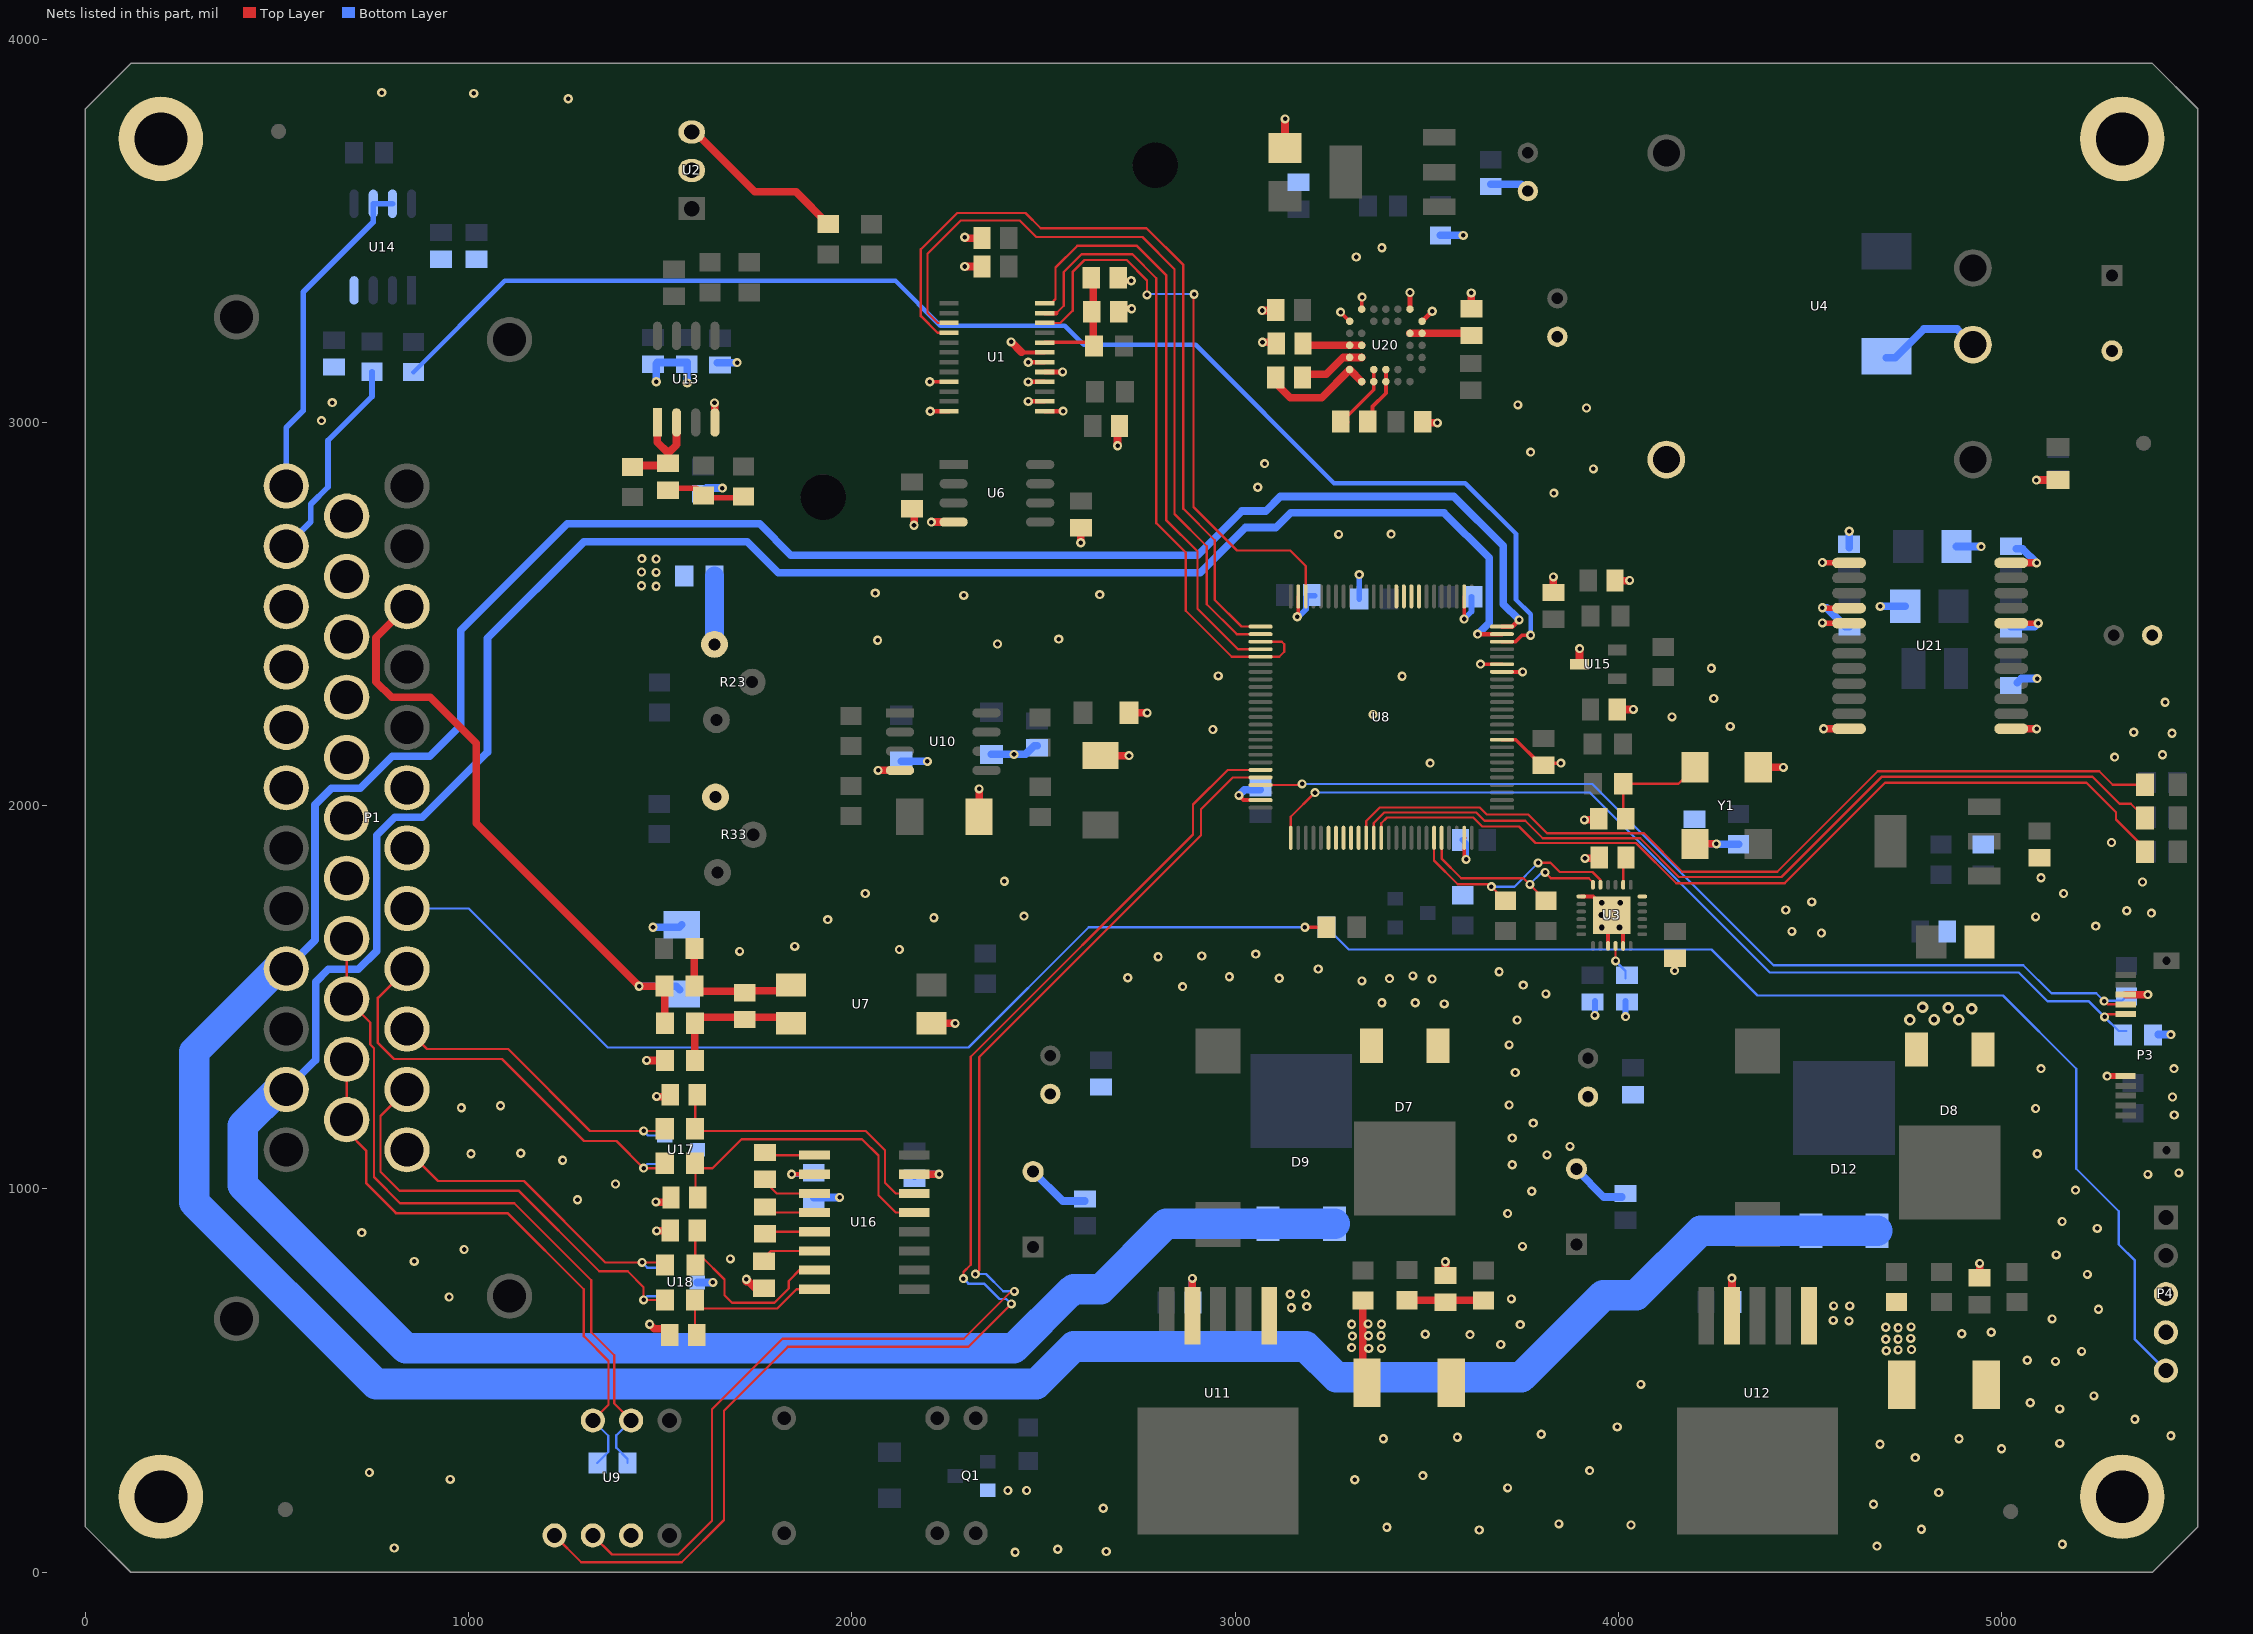
[diagram p0: the nets of this part, all layers, seen from the top]
# Altium PCB MISC82155.PcbDoc (part 3 of 5)
Units mil, origin at the board's own origin, x right, y up, seen from the top; angles counter-clockwise.
Board outline 5511.81 x 3937.01 mil, 4 copper layers (Top Layer, GND, POWER, Bottom Layer); 191 components, 134 nets, 709 pads, 440 vias.

## Via types
v1: diameter 24, hole 12, Top Layer to Bottom Layer, 278 vias
v2: diameter 23.62, hole 11.81, Top Layer to Bottom Layer, 144 vias
v3: diameter 30, hole 15, Top Layer to Bottom Layer, 17 vias
v4: diameter 20, hole 10, Top Layer to Bottom Layer, 1 vias

## Nets (pads, with @x,y where several pads share a name; then routed paths per layer and width w, separated by ;. In a path a pad name is that pad's centre, name@x,y a point inside that pad or via, vN(x,y) a via of type N, cw(c..) or ccw(c..) an arc to the next point about the centre after c; other vN are vias at no path point) (continued)
6050_SCL: R42.1 U3.23 U8.95 | length 630.8
  Top Layer w6: U8.95@3519.2,1916.38 3519.2,1856.8 3581,1795 3662.5,1795 v2(3668.75,1788.75) R42.1@3705.32,1752.18 ; v2(3791,1851) 3823,1851 3847,1827 3933,1827 3953.47,1806.53 U3.23@3953.47,1793.72
  Bottom Layer w6: v2(3668.75,1788.75) 3728.75,1788.75 v2(3791,1851)
6050_SDA: R41.1 U3.24 U8.96 | length 567.4
  Top Layer w6: U8.96@3538.89,1916.38 3538.89,1862.11 3590,1811 3752.5,1811 v2@3768.75,1794.75 ; v2(3769,1795) v2@3768.75,1794.75 ; v2(3809,1826) 3824,1811 3923,1811 3933.79,1800.21 U3.24@3933.79,1793.72 ; R41.1@3811.32,1752.18 v2@3768.75,1794.75
  Bottom Layer w6: v2(3769,1795) 3800,1826 v2(3809,1826)
ACC_INT1: U8.35
ACC_INT2: U8.36
AD_INA: R2.2 U2.3 | length 455.9
  Top Layer w20: U2.3@1582,3758 1591,3758 1747,3602 1854.12,3602 R2.2@1938.41,3517.71
AD_MISO: U1.23 U8.53 U8.55 | length 1728.2
  Top Layer w6: 2533.56,3285.5 2553,3304.93 2553,3393 2599,3439 2732,3439 2794.41,3376.59 2794.41,2737.59 2871,2661 2871,2509 2991.18,2388.82 U8.55@3066.45,2388.82 3115.41,2388.82 3128.41,2401.82 3128.41,2421.34 3121.56,2428.19 U8.53@3066.45,2428.19
  Top Layer w11.81: U1.23@2503.41,3285.5 2533.56,3285.5
AD_MOSI: U1.24 U8.54 | length 1571.4
  Top Layer w6: U1.24@2503.41,3311.09 2520.15,3311.09 2531.41,3322.34 2531.41,3404.41 2588,3461 2744,3461 2820,3385 2820,2746 2902,2664 2902,2514 3007.49,2408.51 U8.54@3066.45,2408.51
AD_NSS: U1.4 U8.51 | length 2102.5
  Top Layer w6: U1.4@2253.41,3234.32 2223.43,3234.32 2180,3277.75 2180,3452 2275,3547 2453,3547 2493,3507 2769,3507 2865,3411 2865,2775 2947,2693 2947,2537 3016.44,2467.56 U8.51@3066.45,2467.56
AD_SCK: U1.3 U8.52 | length 2035.6
  Top Layer w6: U1.3@2253.41,3259.91 2223.84,3259.91 2197.41,3286.34 2197.41,3440.34 2284.07,3527 2438,3527 2481,3484 2758,3484 2842,3400 2842,2761 2926,2677 2926,2526 3004.12,2447.88 U8.52@3066.45,2447.88
AD_SYNC: U1.22 U8.48 | length 1567.8
  Top Layer w6: U1.22@2503.41,3259.91 2543.97,3259.91 2576,3291.93 2576,3393 2607,3424 2717,3424 2770,3371 v1(2770,3333) ; v1@2891.41,3333.41 2891.41,2779.59 3005,2666 3144,2666 3184.56,2625.44 U8.48@3184.56,2546.3
  Bottom Layer w6: v1(2770,3333) 2772.34,3335.34 2892.66,3335.34 v1(2893,3335)
AGND: C3.2 C4.2 C5.2 C11.1 C13.2 C29.2 C30.2 C39.1 C72.2 C73.2 C74.2 C75.2 D4.1 D10.1 D11.1 DW3.1 DW4.1 R4.1 R12.2 R23.1 R33.1 U1.9 U1.12 U1.13 U1.14 U1.16 U1.17 U1.18 U2.2 U6.4 U13.4 U20.F1 U20.G2 | length 1766.4
  Top Layer w10: v1@2204.43,3106.36 U1.9@2253.41,3106.36 ; v1@2460.15,3157.55 v1@2460.41,3157.55
  Top Layer w12: v1(2204.66,3029.59) U1.12@2253.41,3029.59 ; v2(2460.18,3055.18) U1.14@2503.41,3055.18 ; v1@2460.15,3106.36 U1.16@2503.41,3106.36 ; v1@2460.41,3157.55 U1.18@2503.41,3157.55 ; U1.13@2503.41,3029.59 v2(2551.41,3029.59) ; U1.17@2503.41,3131.96 v2(2549.96,3131.96) ; U20.G2@3456.4,3295.83 v1@3456.4,3337.34 ; U20.F1@3487.89,3264.33 v1@3514.15,3290.59
  Top Layer w15: v1@2206,2739 v1(2207.34,2740.34) ; C4.2@2688.93,3297.34 2729.66,3297.34 v1(2730,3297) ; C5.2@2688.93,3370.34 2728.66,3370.34 v1(2729,3370)
  Top Layer w20: v2(1464.34,1335.34) R12.2@1512.04,1335.34 ; v1(1641.41,3051.34) 1642.41,3050.34 U13.4@1642.41,3000.34 ; v1(2162,2732) 2162.41,2732.41 C11.1@2162.41,2780.81 ; v1@2204.41,3029.34 v1(2204.66,3029.59) ; v1(2207.34,2740.34) U6.4@2265.41,2740.34 ; D10.1@2331.96,1971.34 v2(2331.96,2043.96) ; v1(2597.41,2686.34) C13.2@2597.41,2730.81 ; D11.1@2648.41,2130.89 v2(2723.11,2130.89) ; v1@2692.93,2939.81 C3.2@2692.93,2991.34 ; DW4.1@2723.41,2242.34 v2(2770.34,2242.34) ; v1(3070.41,3292.34) C39.1@3113.88,3292.34
  Bottom Layer w20: v2(1481,1683) 1549.45,1683 D4.1@1556,1689.55 ; v1(1489.41,3106.34) 1489.41,3153.81 1492.41,3156.81 1570.41,3156.81 1570.41,3110.34 v2(1570.41,3103.59) ; C72.2@1611,2819.47 1620.53,2829 v2(1662,2829) ; C73.2@1649,3156.47 v2(1700.53,3156.47) ; DW3.1@2129,2116 v2(2197,2116) ; C30.2@2364,2134 v2(2423,2134) 2453,2134 2475.47,2156.47 C29.2@2483,2156.47
  Bottom Layer w50: R23.1@1641.37,2421.23 R4.1@1641.37,2600
  other v1: 2693.41,2939.34 2203.41,3106.34 2460.41,3106.11 2460.41,3157.29 3514.41,3290.34 3456.4,3339.34
ANG_INA: R54.2 U8.23 | length 3611.6
  Top Layer w10: U8.23@3696.37,2428.19 3732.19,2428.19 3749,2445 v2(3771,2445)
  Bottom Layer w12: R54.2@856,3131.63 1094.54,3370.17 2113.83,3370.17 2231,3253 2555,3253 2605,3203 2897,3203 3258,2842 3601,2842 3733,2710 3733,2538 3771,2500 v2(3771,2445)
ANG_R+: P1.24 U14.6 U14.7 | length 880.5
  Bottom Layer w15: P1.24@524.03,2834.48 524.03,2987.03 568,3031 568,3340 751,3523 U14.6@751,3571 U14.7@801,3571
ANG_R-: P1.25 R61.2 | length 548.4
  Bottom Layer w15: P1.25@524.03,2677 588,2740.97 588,2787 633,2832 633,2953 748,3068 R61.2@748,3132.63
AVDD1: C4.1 C5.1 L1.2 U1.20 | length 286.9
  Top Layer w10: U1.20@2504.02,3209.34 L1.2@2630.04,3209.34
  Top Layer w20: L1.2@2629.88,3209.5 2629.88,3297.34 C5.1@2629.88,3370.34
BOOT0: P1.8 P4.5 R34.2 R55.1 | length 5730.9
  Top Layer w10: v2(3182,1683) R55.1@3238.63,1683
  Bottom Layer w6: P1.8@838.99,1732.12 999.88,1732.12 1363,1369 2304,1369 2618,1683 v2(3182,1683) R34.2@3238.63,1683 3296.63,1625 4243,1625 4363,1505 5004,1505 5195,1314 5195,1111 5195,1053 5306,942 5306,855 5348,813 5348,607 P4.5@5429,526
CAN0_RXD: U8.70 U9.1 | length 3518.5
  Top Layer w6: U9.1@1224,96 1294,26 1556,26 1666,136 1666,421 1833,588 2304,588 v2(2416,700) ; v2(2291,766) 2291,783 2310,802 2310,1345 2890,1925 2890,2003 2980.55,2093.55 U8.70@3066.45,2093.55
  Bottom Layer w6: v2(2291,766) 2304,753 2345,753 2385,713 2403,713 v2(2416,700)
CAN0_TXD: U8.71 U9.2 | length 3345.1
  Top Layer w6: U9.2@1324,96 1374,46 1547,46 1635,134 1635,425 1819,609 2292,609 2416,733 v2(2424,733) ; v2(2322,778) 2322,777 2332,787 2332,1344 2911,1923 2911,1991 2993.86,2073.86 U8.71@3066.45,2073.86
  Bottom Layer w6: v2(2322,778) 2350,778 2395,733 v2(2424,733)
CANH: P1.22 P1.23 R40.1 U9.7 | length 1566.3
  Top Layer w6: P1.22@681.51,1338.42 P1.23@681.51,1180.94 681.51,1150.49 733,1099 733,1014 810,937 1101,937 1300,738 1300,665 ; 1300,651 1300,665 ; U9.7@1324,396 1365,437 1365,551 1300,616 1300,665
  Bottom Layer w6: U9.7@1324,396 1364,356 1364,313.37 R40.1@1335.63,285
CANL: P1.20 P1.21 R40.2 U9.6 | length 1878.8
  Top Layer w6: P1.20@681.51,1653.38 P1.21@681.51,1495.9 743,1434.41 743,1377 753,1367 753,1031 821,963 1119,963 1320,762 1320,626 1380,566 1380,440 U9.6@1424,396
  Bottom Layer w6: R40.2@1414.37,285 1414.37,295.63 1385,325 1385,357 U9.6@1424,396
COM1_RXD: P1.11 R59.2 U18.1 | length 1203
  Top Layer w6: P1.11@838.99,1259.68 770,1190.69 770,1045 820,995 1131,995 1341,785 1415,785 1456.34,743.66 v2(1456.34,710.34) R59.2@1512.04,710.34
  Bottom Layer w6: v2(1456.34,710.34) 1465.94,719.94 U18.1@1511.91,719.94
COM1_TXD: P1.12 R58.2 U18.2 | length 860
  Top Layer w6: P1.12@838.99,1102.2 920.19,1021 1144,1021 1356.66,808.34 v2(1452.34,808.34) R58.2@1512.04,808.34
  Bottom Layer w6: v2(1452.34,808.34) 1465.94,794.74 U18.2@1511.91,794.74
COM2_RXD: P1.9 R57.2 U17.1 | length 1169.4
  Top Layer w6: P1.9@838.99,1574.64 763,1498.65 763,1381 805,1339 1087,1339 1301,1125 1385.68,1125 v2(1456.34,1054.34) R57.2@1512.04,1054.34
  Bottom Layer w6: v2(1456.34,1054.34) 1466.94,1064.94 U17.1@1511.91,1064.94
COM2_TXD: P1.10 R56.2 U17.2 | length 843.5
  Top Layer w6: P1.10@838.99,1417.16 891.15,1365 1103,1365 1316.66,1151.34 v2(1456.34,1151.34) R56.2@1512.04,1151.34
  Bottom Layer w6: v2(1456.34,1151.34) 1467.94,1139.74 U17.2@1511.91,1139.74
FOOT_SW: D4.2 P1.3 R6.1 R8.1 | length 1653.8
  Top Layer w20: P1.3@853.48,2519.52 P1.3@838.99,2519.52 758,2438.53 758,2324 799,2283 900,2283 1020,2163 1020,1954 v2@1444.66,1529.34 ; v2(1445,1529) v2@1444.66,1529.34 ; R8.1@1511.04,1529.34 v2@1444.66,1529.34 ; R6.1@1512.04,1432.34 R8.1@1512.04,1528.34
  Bottom Layer w20: v2(1445,1529) 1541.3,1529 D4.2@1550.41,1519.89
GND: C1.2 C6.2 C7.1 C8.2 C9.1 C10.2 C12.1 C14.2 C15.2 C17.1 C18.2 C19.2 C21.2 C22.2 C23.2 C24.2 C25.2 C26.2 C27.2 C28.1 C31.2 C32.2 C33.2 C34.2 C35.2 C36.1 C37.1 C40.2 C41.1 C42.1 C43.2 C44.1 C46.2 C47.2 C48.2 C50.2 C51.2 C52.2 C53.2 C54.1 C55.1 C56.1 C57.2 C61.2 C62.2 C63.2 C64.2 C65.2 C66.2 C67.2 C68.2 C69.2 C70.1 C76.2 C77.2 C78.2 D5.2 D6.1 D7.1 D8.1 H1.8 H2.8 H3.8 H4.8 P1.6 P1.7 P1.13 P1.14 P1.15 P1.16 P1.17 P1.18 P1.19 P1.26 P1.27 P1.28 P1.29 P3.5 P3.8 P4.3 P4.4 Q1.2 R4.2 R13.1 R20.1 R21.1 R27.1 R28.1 R38.1 R44.1 U1.19 U3.1 U3.9 U3.11 U3.18 U4.2 U4.5 U7.3 U8.10 U8.19 U8.20 U8.27 U8.49 U8.74 U8.99 U9.3 U10.4 U11.1 U12.1 U14.4 U15.3 U16.15 U17.3 U18.3 U20.F7 U20.G6 U21.1 U21.8 U21.12 U21.13 U21.16 U21.17 U21.24 Y1.2 | length 4636.4
  Top Layer w6: v2(3597.41,2487.34) v2@3597.94,2487.88
  Top Layer w9: v2@3597.94,2487.88 U8.27@3597.94,2546.3
  Top Layer w10: 2442.61,3183.14 U1.19@2503.41,3183.14 ; v2(3010,2027) 3022.19,2014.81 U8.74@3066.45,2014.81 ; v1(3162.41,2493.34) 3162.41,2496.34 3164.87,2498.81 U8.49@3164.87,2546.3 ; v1@3275.41,3287.85 U20.F7@3298.92,3264.33 ; U20.G6@3330.41,3295.83 v1@3330.41,3326.35 ; U8.99@3598.41,1915.92 U8.99@3597.94,1916.38 3597.94,1865.06 v2(3603,1860) ; v2(3640.41,2369.34) 3640.61,2369.14 U8.20@3696.37,2369.14 ; U8.10@3696.37,2172.29 3732.46,2172.29 3793.93,2110.81 3849.88,2110.81 v2(3850.41,2111.34) ; U8.19@3696.37,2349.45 3750.3,2349.45 v2(3750.41,2349.34) ; U3.1@3903.28,1763.21 3933.79,1763.21 U3.1@3983,1714 3973.16,1704.16 U3.9@3973.16,1634.28 ; U3.11@4012.53,1634.28 U3.1@4012.53,1684.47
  Top Layer w15: U3.1@3983,1714 U3.1@4012.53,1684.47 ; v2(4147,1570) 4147,1606.47 C41.1@4148,1607.47 ; v1@4533.61,2476.35 U21.17@4602.17,2476.35 ; v1@4533.61,2515.72 U21.16@4602.17,2515.72 ; v1@4533.61,2633.83 U21.13@4602.17,2633.83 ; U21.8@5025.4,2476.35 v1(5095.66,2476.41) ; v2(5275.35,1294.65) P3.5@5323.46,1294.65
  Top Layer w20: v2(1472,647) 1484,635 C50.2@1535,635 ; v2(1488.41,966.34) 1489.41,965.34 C52.2@1532.88,965.34 ; v2(1490.41,890.34) 1491.41,891.34 C51.2@1531.88,891.34 ; v2(1490.41,1241.34) 1491.41,1240.34 C53.2@1531.88,1240.34 ; v2@1724.93,758.34 v2@1730.41,758.34 ; v2@1724.93,763.81 v2(1724.41,764.34) v2@1730.41,758.34 ; C48.2@1771,741 1747.75,741 v2@1730.41,758.34 ; v2(2068.34,2092.34) U10.4@2125.41,2092.34 ; U16.15@2162.41,1038.34 v2(2227.41,1038.34) ; U7.3@2207.48,1432.34 v2(2269.41,1432.34) ; v1@2295.41,3481.34 C14.2@2344.88,3481.34 ; v1@2296.41,3407.34 C15.2@2344.88,3407.34 ; v1(2415.41,3210.34) 2442.61,3183.14 ; v1@3072.41,3209.34 C56.1@3114.88,3209.34 ; C6.2@3130.41,3716.33 v1@3130.41,3791.34 ; C44.1@3483.93,2999.34 v2(3527.66,2999.34) ; C32.2@3549,768.53 v2(3549,810) ; C57.2@3616.41,3291.87 v1(3616.41,3338.34) ; C37.1@3830.41,2550.87 v2(3830.41,2597.34) ; U15.3@3898.79,2369 v2(3898.79,2409.79) ; v2(3911.41,1963.34) C28.1@3954.88,1963.34 ; v2(3913.07,1862.75) C55.1@3955.54,1862.75 ; C36.1@3985.93,2587.34 4028.41,2587.34 v2(4029.41,2588.34) ; C17.1@3991.93,2251.34 v2(4039.41,2251.34) ; Y1.2@4365.08,2100.34 v2(4430.66,2100.34) ; v2(4536,2201) 4536.24,2200.76 U21.24@4602.17,2200.76 ; C69.2@4943,762.53 v2(4943,806) ; U21.1@5025.4,2200.76 v2(5091.76,2200.76) ; U21.12@5025.4,2633.83 v2(5091.83,2633.83) ; v2(5091.03,2850.03) D5.2@5147.41,2850.03 ; P3.8@5324.16,1507.25 v2(5381.75,1507.25)
  Bottom Layer w15: v1(3162.41,2493.34) 3165.34,2493.34 3185,2513 3185,2544 3189.34,2548.34 C27.2@3207.93,2548.34 ; R20.1@3324.04,2539.34 v2(3324.04,2602.96) ; C26.2@3593.47,1911 3603,1901.47 v2(3603,1860) ; v2(3597.41,2487.34) 3616.93,2506.87 C24.2@3616.93,2545.34 ; v2(3939,1453) C42.1@3939,1490.47 ; v2(4019,1450) C54.1@4019,1490.47
  Bottom Layer w20: U18.3@1596.5,756 v2(1637,756) ; C47.2@1900.41,977.81 v2(1968.19,977.81) ; C46.2@2163.41,1033.81 2167.93,1038.34 v2(2227.41,1038.34) ; C18.2@2473,1045.43 2549.9,968.53 C19.2@2608,968.53 ; v2(3010,2027) 3024.53,2041.53 C25.2@3066,2041.53 ; R21.1@3536,3488.63 v2(3595.37,3488.63) ; C7.1@3667,3621.47 3746.53,3621.47 C1.2@3764,3604 ; C33.2@3891,1052.43 3891,1049.87 3962,978.87 C34.2@4009.41,978.87 ; v1(4532.66,2516.67) 4543.33,2516.67 4593,2467 C65.2@4603,2467 ; C63.2@4602.66,2672.93 v2(4602.66,2716.34) ; v2(4683.59,2520.41) C62.2@4748.67,2520.41 ; D6.1@4700,3169.19 4722.19,3169.19 4797,3244 4884.75,3244 U4.2@4925.41,3203.34 ; C61.2@4882.65,2676.41 v2(4946.59,2676.41) ; C64.2@5024.66,2466.88 5086.13,2466.88 v1(5095.66,2476.41) ; C66.2@5038.73,2671 5054.66,2671 v2(5091.83,2633.83) ; C67.2@5041,2321 5051.88,2331.88 v2(5092.88,2331.88) ; R44.1@5409.37,1403 v2(5442,1403)
  other v1: 2426,52 2664,54 2537,60 806,63 4675,68 5159,73 3637,110 4791,112 3396,117 4033,123 3845,126 2656,167 4666,177 4836,208 2407,213 2456,213 3711,220 3312,241 952,242 3490,252 741,260 3925,265 4775,299 5000,322 4683,334 5152,336 3387,348 4889,348 3580,352 5442,356 3799,360 3997,379 5348,399 5152,426 5075,442 5241,460 4059,490 5141,550 5067,553 5209,576 3693,594 3613,620 3496,621 4896,622 4973,626 3744,646 4561,657 5132,661 5253,686 3147,690 3187,693 3721,713 949,718 3144,725 3184,726 5224,777 858,811 5143,828 988,842 3750,850 721,886 5250,897 5158,915 3711,936 1284,972 3774,994 5193,997 1383,1013 5382,1038 5463,1042 3723,1063 1245,1075 3814,1089 1006,1092 5093,1092 1136,1093 3874,1111 3723,1133 3778,1172 5451,1193 5089,1210 981,1212 1083,1217 3715,1219 5446.19,1240 3731,1304 5103,1314 5450.19,1314 3715,1376 3736,1441 3546,1483 3383,1486 3470,1486 3811,1509 2863,1528 3752,1532 3331,1543 3514,1548 3403,1549 3115,1550 2720,1551 2985,1554 3464,1556 3689,1567 3217,1574 2799,1606 2913,1608 3054,1613 1707,1620 2124,1625 1851,1633 4530,1668 4453,1672 5246,1686 1937,1703 2214,1708 5089,1710 2449,1712 5391,1720 5327,1726 4437,1728 4505,1749 2035,1771 5162,1771 5368,1801 2398,1803 5103,1812 5287,1904 5295,2127 5420,2133 5445,2189 5345,2192 2942,2199 4292,2207 4140,2232 5427,2270 4249,2280 2956,2339 4243,2359 2380,2422 2067,2432 2540,2435 4532.66,2477.3 2292,2549 2647,2551 2061,2555 1489,2573 1451,2574 1489,2609 1451,2610 4532.66,2634.78 1489,2644 1452,2645 3270,2708 3407,2709 3832,2816 3059,2831 3935,2879 3077,2893 3771,2923 616,3005 3917,3038 3738,3046 644,3052 3071.41,3209.34 3275.41,3288.34 3331.41,3327.34 2294.41,3407.34 3316,3432 3383,3456 2294.41,3483.34 3130.41,3792.34 1260,3845 1013,3859 773,3861
  other v2: 4602,656 4562,695 4604,695 1682.93,817.81 3509,2111 3360,2238 3436,2338
  other v3: 4761,1441 4889,1441 4824,1442 4922,1470 4861,1473 4794,1474 3957,1682 4003,1682 3956,1715 3957,1747 4005,1747
GND_SA: D9.1 P1.34 R13.2 R16.1 U8.24 | length 8267.6
  Top Layer w12: v2(3633.12,2447.88) U8.24@3696.37,2447.88
  Top Layer w20: R13.2@3333.17,532.34 R16.1@3333.17,707.8
  Bottom Layer w20: P1.34@524.03,1259.68 601,1336.65 601,1540 634,1573 712,1573 760,1621 760,1923 807,1970 879,1970 1049,2140 1049,2437 1301,2689 1727,2689 1808,2608 2909,2608 3027,2726 3106,2726 3145,2765 3545,2765 3663,2647 3663,2477.75 v2(3633.12,2447.88)
  Bottom Layer w80: P1.34@524.03,1259.68 504.68,1259.68 410,1165 410,1010 836,584 2422,584 2570,732 2572.02,732 2578.52,738.5 2649.5,738.5 2820,909 D9.1@3086.39,909 D9.1@3259.61,909
  other v1: 3349,584 3382,584 3304,586 3306,616 3348,617 3381,617 3304,647 3382,647 3347,648
GND_SB: D12.1 P1.32 R26.1 R27.2 U8.25 | length 10109
  Top Layer w12: U8.25@3696.37,2467.56 3723.56,2467.56 v2(3741,2485)
  Bottom Layer w20: P1.32@524.03,1574.64 599.08,1649.7 599.08,1920.69 599,1920.77 599,2003 642,2046 717,2046 800.51,2129.51 898.51,2129.51 979,2210 979,2458 1257,2736 1759,2736 1841,2654 2902,2654 3017,2769 3080,2769 3118,2807 3571,2807 3700,2678 3700,2526 v2(3741,2485)
  Bottom Layer w80: P1.32@524.03,1574.64 500.64,1574.64 284,1358 284,965 758,491 2481,491 2579,589 3184,589 3264,509 3531,509 ; 3675.34,509 3531,509 ; D12.1@4675.61,891 D12.1@4502.39,891 4215,891 4047,723 3961,723 3747,509 3531,509
  other v1: 4699,578 4730,580 4765,581 4698,608 4730,608 4763,610 4730,638 4698,639 4764,640
GYRO_INT1: U8.34
GYRO_INT2: U8.33
JTCK: P3.6 R44.2 U8.76 | length 2577.8
  Top Layer w6: U8.76@3145.19,1916.38 3145.19,1971.19 v2(3208.5,2034.5) ; v2(5269,1449) 5276.07,1456.07 P3.6@5324.16,1456.07
  Bottom Layer w6: v2(3208.5,2034.5) 3925.5,2034.5 4395,1565 5045,1565 5120.5,1489.5 5228.5,1489.5 v2(5269,1449) 5306,1412 R44.2@5326,1412
JTMS: P3.7 R45.2 U8.72 | length 2549.2
  Top Layer w6: U8.72@3066.45,2054.18 3164.18,2054.18 3167,2057 v2(3175,2057) ; v2@5276.34,1481.66 P3.7@5324.16,1481.66
  Bottom Layer w6: v2(3175,2057) 3932,2057 4405,1584 5057,1584 5130.5,1510.5 5247.5,1510.5 v2@5267,1491 ; v2(5268,1490) v2@5267,1491 ; R45.2@5326,1502.63 5314.37,1491 v2@5267,1491
LED_O1: D1.2 U8.88 | length 2307.4
  Top Layer w6: U8.88@3381.41,1916.38 3381.41,1954.34 3396.41,1969.34 3621.41,1969.34 3644.75,1946 3741,1946 3784,1903 4046,1903 4151,1798 4434,1798 4696,2060 5222,2060 5299,1983 5299,1964 5374.39,1888.61 D1.2@5374.39,1880
LED_O2: D2.2 U8.87 | length 2285.4
  Top Layer w6: U8.87@3361.72,1916.38 3361.72,1954.66 3389.41,1982.34 3629.41,1982.34 3650.75,1961 3757,1961 3803,1915 4057,1915 4158,1814 4426,1814 4688,2076 5237,2076 5308,2005 5337.39,2005 D2.2@5374.39,1968
LED_O3: D3.2 U8.86 | length 2282.9
  Top Layer w6: U8.86@3342.04,1916.38 3342.04,1959.97 3377.41,1995.34 3638.41,1995.34 3656.75,1977 3765,1977 3814,1928 4067,1928 4167,1828 4415,1828 4677,2090 5255,2090 5290,2055 D3.2@5374.39,2055
LED_O4: U8.85
LED_O5: U8.84
LED_O6: U8.83
LED_O7: U8.82
LED_O8: U8.81
NetC2_1: C2.1 R39.1 U13.1 U13.2 | length 319
  Top Layer w20: R39.1@1416,2884.37 1419.5,2887.87 C2.1@1520.41,2887.87 ; U13.1@1492.41,3000.34 1492.41,2948.59 1520.41,2920.59 ; C2.1@1520.25,2887.71 C2.1@1520.41,2887.87 ; U13.2@1542.41,3000.34 1542.41,2942.59 1520.41,2920.59 ; C2.1@1520.41,2887.87 1520.41,2920.59
NetC2_2: C2.2 R43.2 R46.1 | length 239.1
  Top Layer w11.81: R46.1@1588.56,2828.81 R46.1@1609.41,2807.97 ; R43.2@1708.41,2807.97 R43.2@1709.41,2806.97
  Top Layer w15: C2.2@1520.41,2828.81 1593.82,2828.81 1618.94,2803.69 1714.06,2803.69 R43.2@1717,2806.63
NetC16_1: C16.1 R8.2 R11.1 U7.1 | length 369.8
  Top Layer w19.68: R11.1@1588.78,1627.34 1588.78,1530.34 1602.78,1516.34 1710.93,1516.34 1720.41,1506.87 1730.88,1517.34 1826.34,1517.34 U7.1@1841.34,1532.34
NetC16_2: C16.2 R6.2 R12.1 U7.2 | length 364
  Top Layer w19.68: R12.1@1590.78,1331.34 1589.78,1332.34 1589.78,1429.34 1608.25,1447.81 1825.86,1447.81 U7.2@1841.34,1432.34
NetC20_2: C20.2 U11.4 | length 178.3
  Top Layer w9.84: U11.4@2888.48,669.34 U11.4@2888.48,686.34
  Top Layer w20: U11.4@2888.48,669.34 v2(2888.48,766.52)
  Bottom Layer w20: C20.2@2884.53,704 2888.48,707.95 v2(2888.48,766.52)
NetC22_1: C22.1 L2.1 Y1.4 | length 171.3
  Top Layer w19.68: Y1.4@4199.73,1900.34 v2(4255.66,1900.34)
  Bottom Layer w19.68: C22.1@4199,1900.47 4199.13,1900.34 v2(4255.66,1900.34) 4256.37,1899.63 L2.1@4314,1899.63
NetC28_2: C28.2 R36.2 Y1.3 | length 299.2
  Top Layer w6: C28.2@4013.93,1963.34 4012.78,1964.5 R36.2@4012.78,2057.34 4156.73,2057.34 Y1.3@4199.73,2100.34
NetC32_1: C32.1 R14.2 R30.2 | length 199.4
  Top Layer w20: R14.2@3449,709.63 3647,709.63 R30.2@3648,708.63
NetC38_2: C38.2 U12.4 | length 161.9
  Top Layer w20: U12.4@4296.48,669.34 v2(4296.48,767.52)
  Bottom Layer w20: C38.2@4293.53,705 4296.48,707.95 v2(4296.48,767.52)
NetC45_1: C45.1 U16.3 | length 141.6
  Top Layer w6: C45.1@1773.41,1018.81 1803.88,988.34 U16.3@1902.41,988.34
NetC45_2: C45.2 U16.1 | length 133.3
  Top Layer w6: C45.2@1773.41,1077.87 1783.88,1088.34 U16.1@1902.41,1088.34
NetC47_1: C47.1 U16.2 | length 157.5
  Top Layer w6: U16.2@1902.41,1038.34 U16.2@1939.41,1038.34
  Top Layer w12: v2(1842.66,1038.34) U16.2@1902.41,1038.34
  Bottom Layer w12: v2@1841,1040 v2(1842.66,1038.34) 1844.13,1036.87 C47.1@1900.41,1036.87
NetC48_1: C48.1 U16.6 | length 135.4
  Top Layer w6: C48.1@1773.41,822.87 1788.88,838.34 U16.6@1902.41,838.34
NetC49_1: C49.1 U16.5 | length 130.5
  Top Layer w6: C49.1@1773.41,884.81 1776.93,888.34 U16.5@1902.41,888.34
NetC49_2: C49.2 U16.4 | length 131.3
  Top Layer w6: C49.2@1773.41,943.87 1778.93,938.34 U16.4@1902.41,938.34
NetC50_1: C50.1 R59.1 U16.8 | length 394.5
  Top Layer w6: C50.1@1589.93,626.34 1590.78,627.18 1590.78,688 1805,688 1855.34,738.34 U16.8@1902.41,738.34
NetC51_1: C51.1 R58.1 U16.7 | length 522.1
  Top Layer w6: C51.1@1590.93,891.34 1590.93,808.5 1606.72,824.28 1667.5,763.5 1667.5,722.5 1687,703 1798,703 1835.03,740.03 1835.03,759.97 1863.41,788.34 U16.7@1902.41,788.34
NetC52_1: C52.1 R57.1 U16.13 | length 832.6
  Top Layer w6: C52.1@1591.93,965.34 1591.93,1053.18 1590.78,1054.34 1636.41,1054.34 1712.07,1130 2026.41,1130 2069.41,1087 2069.41,983.34 2114.41,938.34 U16.13@2162.41,938.34
NetC53_1: C53.1 R56.1 U16.14 | length 777.8
  Top Layer w6: C53.1@1590.93,1240.34 1590.93,1151.5 1590.78,1151.34 2036.07,1151.34 2086.41,1101 2086.41,1016.34 2114.41,988.34 U16.14@2162.41,988.34
NetC54_2: C54.2 U3.10 | length 95.6
  Top Layer w6: v2(3992.84,1595.16) U3.10@3992.84,1634.28
  Bottom Layer w6: v2(3992.84,1595.16) 4019,1569 C54.2@4019,1549.53
NetC55_2: C55.2 U3.20 | length 98.1
  Top Layer w6: U3.20@4012.53,1793.72 C55.2@4012.53,1877 ; C55.2@4013.59,1856.75 C55.2@4024.07,1846.28
NetC56_2: C56.2 U20.D6 U20.D7 | length 276.8
  Top Layer w10: C56.2@3181.93,3201.34 U20.D7@3298.92,3201.34
  Top Layer w20: C56.2@3173.93,3209.34 3181.93,3201.34 U20.D7@3298.92,3201.34 U20.D6@3330.41,3201.34
NetC57_1: C57.1 U20.E1 U20.E2 | length 160
  Top Layer w20: U20.E2@3456.4,3232.84 U20.E1@3487.89,3232.84 C57.1@3616.38,3232.84
NetC58_1: C58.1 U20.A6 U20.B7 | length 318.4
  Top Layer w20: C58.1@3115.47,3129 3115.47,3093.53 3144,3065 3225.57,3065 U20.B7@3298.92,3138.35 U20.A6@3330.41,3106.85 ; C58.1@3116.47,3120.22 C58.1@3116.47,3133
NetC58_2: C58.2 U20.C6 U20.C7 | length 175.9
  Top Layer w20: C58.2@3175.53,3133 3182.53,3126 3238.07,3126 3281.91,3169.85 U20.C7@3298.92,3169.85 U20.C6@3330.41,3169.85
NetC59_1: C59.1 U20.A5 U20.B5 | length 170.9
  Top Layer w10: C59.1@3285,3001 3285,3008.74 3361.91,3085.65 U20.A5@3361.91,3106.85 U20.B5@3361.91,3138.35 ; C59.1@3293.88,2999.34 C59.1@3293.88,3001
NetC59_2: C59.2 U20.A4 U20.B4 | length 161.8
  Top Layer w10: C59.2@3352.93,2999.34 C59.2@3360,3006.41 ; C59.2@3358.53,3001 3358.53,3041.53 3393.41,3076.41 U20.A4@3393.41,3106.85 U20.B4@3393.41,3138.35